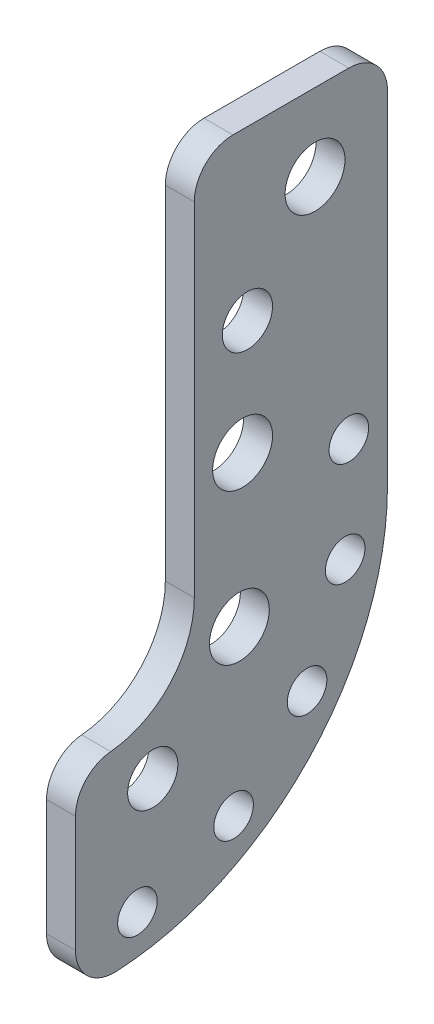
SolidWorks part; units mm, degrees
material "Thornel Mat VMA"
ref_plane "前视基准面" through (0, 0, 0) normal (0, 0, 1) x (1, 0, 0)
ref_plane "上视基准面" through (0, 0, 0) normal (0, 1, 0) x (1, 0, 0)
ref_plane "右视基准面" through (0, 0, 0) normal (1, 0, 0) x (0, 0, -1)
sketch "草图1" plane through (0, 0, 0) normal (1, 0, 0) x (0, 0, -1)
  line L0 (0, 0) -> (0, 48.25) construction
  line L1 (-9.25, 0) -> (-9.25, 19.75)
  line L2 (9.25, 0) -> (9.25, 19.75)
  line L3 (-24, -33.25) -> (-24, -37.75)
  line L4 (9.25, 19.75) -> (19.25, 19.75)
  line L5 (19.25, 19.75) -> (19.25, 0)
  line L6 (-24, -37.75) -> (6.7494, -37.75)
  line L7 (-24, -4.75) -> (-25.4, -4.75)
  line L8 (-25.4, -4.75) -> (-25.4, -14.75)
  line L9 (-25.4, -14.75) -> (-24, -14.75)
  line L10 (-19.25, 0) -> (-19.25, 19.75)
  line L11 (-19.25, 19.75) -> (-9.25, 19.75)
  line L12 (-24, 0) -> (11.1869, -2.1081) construction
  line L13 (-24, 0) -> (10.4888, -7.2859) construction
  line L14 (11.25, 3.1162) -> (11.25, 0) construction
  line L15 (-11.25, 0) -> (-11.25, 3.1162) construction
  line L16 (-24, 0) -> (-11.4381, -2.1822) construction
  line L17 (-24, 0) -> (-13.4117, -7.1029) construction
  line L18 (-24, -33.25) -> (-24, -14.75) construction
  line L19 (14, -37.75) -> (14, -27.25) construction
  line L20 (14, -27.25) -> (19.25, -27.25) construction
  line L21 (-24, 0) -> (-44, 0) construction
  line L22 (11.25, 3.1162) -> (11.1869, -2.1081) construction
  line L23 (10.4888, -7.2859) -> (11.1869, -2.1081) construction
  line L24 (-11.25, 3.1162) -> (-11.4381, -2.1822) construction
  line L25 (-11.4381, -2.1822) -> (-13.4117, -7.1029) construction
  line L26 (-25.4, -9.75) -> (-24, -9.75)
  line L27 (-14.25, 0) -> (-14.25, 19.75)
  line L28 (14.25, 0) -> (14.25, 19.75)
  line L29 (-17.8356, -34.7068) -> (-17.8356, -37.75) construction
  line L30 (-19.25, 19.75) -> (-19.25, 48.25)
  line L31 (-19.25, 48.25) -> (-9.25, 48.25)
  line L32 (19.25, 48.25) -> (19.25, 19.75)
  line L33 (9.25, 19.75) -> (9.25, 48.25)
  line L34 (-9.25, 19.75) -> (-9.25, 48.25)
  line L35 (9.25, 48.25) -> (19.25, 48.25)
  line L36 (-24, 0) -> (-1.8285, -34.25) construction
  line L37 (-24, 0) -> (16.5703, -4.3237) construction
  line L38 (-24, 0) -> (10.7567, -21.3684) construction
  line L39 (16.5703, -4.3237) -> (14.6157, -13.1708) construction
  line L40 (14.6157, -13.1708) -> (10.7567, -21.3684) construction
  line L41 (-14.25, 6.1162) -> (14.25, 6.1162)
  arc A0 (-24, -24) -> (0, 0) centre (-24, 0) ccw construction
  arc A1 (-24, -33.25) -> (9.25, 0) centre (-24, 0) ccw
  arc A2 (-24, -14.75) -> (-9.25, 0) centre (-24, 0) ccw
  arc A3 (6.7494, -37.75) -> (19.25, 0) centre (-44, 0) ccw
  arc A4 (-24, -4.75) -> (-19.25, 0) centre (-24, 0) ccw
  circle A5 centre (11.1869, -2.1081) radius 1.025
  circle A6 centre (10.4888, -7.2859) radius 1.025
  circle A7 centre (9.0331, -12.3036) radius 1.025
  circle A8 centre (6.8516, -17.0511) radius 1.025
  circle A9 centre (3.9925, -21.4239) radius 1.025
  circle A10 centre (0.5183, -25.3262) radius 1.025
  circle A11 centre (-3.4944, -28.672) radius 1.025
  circle A12 centre (-7.9577, -31.388) radius 1.025
  circle A13 centre (11.1869, -2.1081) radius 2.5 construction
  circle A14 centre (10.4888, -7.2859) radius 2.5 construction
  circle A15 centre (11.25, 3.1162) radius 1.025
  circle A16 centre (11.25, 3.1162) radius 2.5 construction
  arc A17 (11.25, 0) -> (-7.9577, -31.388) centre (-24, 0) cw construction
  arc A18 (-11.25, 0) -> (-22.1936, -12.6214) centre (-24, 0) cw construction
  circle A19 centre (-11.4381, -2.1822) radius 1.025
  circle A20 centre (-11.4381, -2.1822) radius 2.5 construction
  circle A21 centre (-13.4117, -7.1029) radius 1.025
  circle A22 centre (-17.2162, -10.7955) radius 1.025
  circle A23 centre (-22.1936, -12.6214) radius 1.025
  circle A25 centre (-11.25, 3.1162) radius 1.025
  circle A26 centre (-11.25, 3.1162) radius 2.5 construction
  circle A27 centre (-13.4117, -7.1029) radius 2.5 construction
  circle A28 centre (8, -29.75) radius 1.55
  circle A29 centre (9.0331, -12.3036) radius 2.5 construction
  circle A30 centre (6.8516, -17.0511) radius 2.5 construction
  circle A31 centre (3.9925, -21.4239) radius 2.5 construction
  circle A32 centre (0.5183, -25.3262) radius 2.5 construction
  circle A33 centre (-3.4944, -28.672) radius 2.5 construction
  circle A34 centre (-7.9577, -31.388) radius 2.5 construction
  circle A35 centre (-17.2162, -10.7955) radius 2.5 construction
  circle A36 centre (-22.1936, -12.6214) radius 2.5 construction
  arc A37 (-24, -9.75) -> (-14.25, 0) centre (-24, 0) ccw
  arc A38 (-17.8356, -37.75) -> (14.25, 0) centre (-24, 0) ccw
  arc A39 (-24, -38.25) -> (14.25, 0) centre (-24, 0) ccw construction
  circle A40 centre (-12.7733, -33.4144) radius 1.025
  circle A41 centre (-17.8356, -34.7068) radius 1.025
  circle A42 centre (-12.7733, -33.4144) radius 2.5 construction
  circle A43 centre (-17.8356, -34.7068) radius 2.5 construction
  circle A44 centre (-21.4, -7.0349) radius 1.3
  circle A45 centre (-16.9174, -2.467) radius 1.55
  arc A48 (-16.9174, -2.467) -> (-21.4, -7.0349) centre (-24, 0) cw construction
  arc A49 (16.5703, -4.3237) -> (-1.8285, -34.25) centre (-24, 0) cw construction
  circle A50 centre (16.5703, -4.3237) radius 1.3
  circle A51 centre (14.6157, -13.1708) radius 1.55
  circle A52 centre (10.7567, -21.3684) radius 1.3
  circle A53 centre (-1.8285, -34.25) radius 1.3
  circle A55 centre (16.75, 5.25) radius 1.55
  circle A56 centre (-16.75, 5.25) radius 1.55
  circle A57 centre (-13, 15.75) radius 1.55
  circle A58 centre (-13, 15.75) radius 2.5 construction
  circle A59 centre (13, 15.75) radius 1.55
  circle A60 centre (13, 15.75) radius 2.5 construction
  circle A61 centre (-16.5, 11.05) radius 1.3
  circle A62 centre (16.5, 11.05) radius 1.3
  point P120 (0, 0)
  point P121 (0, 0)
  dimension "D1" = 24
  dimension "D2" = 18.5
  dimension "D4" = 10
  dimension "D5" = 1.4
  dimension "D6" = 10
  dimension "D8" = 2.05
  dimension "D10" = 5
  dimension "D11" = 4
  dimension "D13" = 12.75
  dimension "D15" = 3.5
  dimension "D16" = 3.1
  dimension "D18" = 6
  dimension "D23" = 53
  dimension "D24" = 2.6
  dimension "D25" = 3.1
  dimension "D26" = 7.5
  dimension "D33" = 40.8
  dimension "D28" = 6.4
  dimension "D32" = 5
  dimension "D34" = 26
  dimension "D3" = 4.5
  dimension "D7" = 8.5
  dimension "D9" = 35.25
  dimension "D12" = 24
  dimension "D14" = 24.5
  dimension "D17" = 8
  dimension "D19" = 2.5
  dimension "D20" = 20
  dimension "D21" = 5
  dimension "D27" = 4
  dimension "D29" = 2.5
  dimension "D30" = 14.5
  dimension "D31" = 32
  dimension "D35" = 51
  dimension "D36" = 3
  dimension "D37" = 4
  dimension "D38" = 5.8
  dimension "D39" = 33
  dimension "D22" = 5
extrude "凸台-拉伸1" add sketch "草图1" along normal blind 1.5
fillet "R2 圆角1" radius 2 4 edges at (0.75, 19.75, 19.25) (0.75, 19.75, 9.25) (0.75, -4.75, 25.4) (0.75, -14.75, 25.4)
